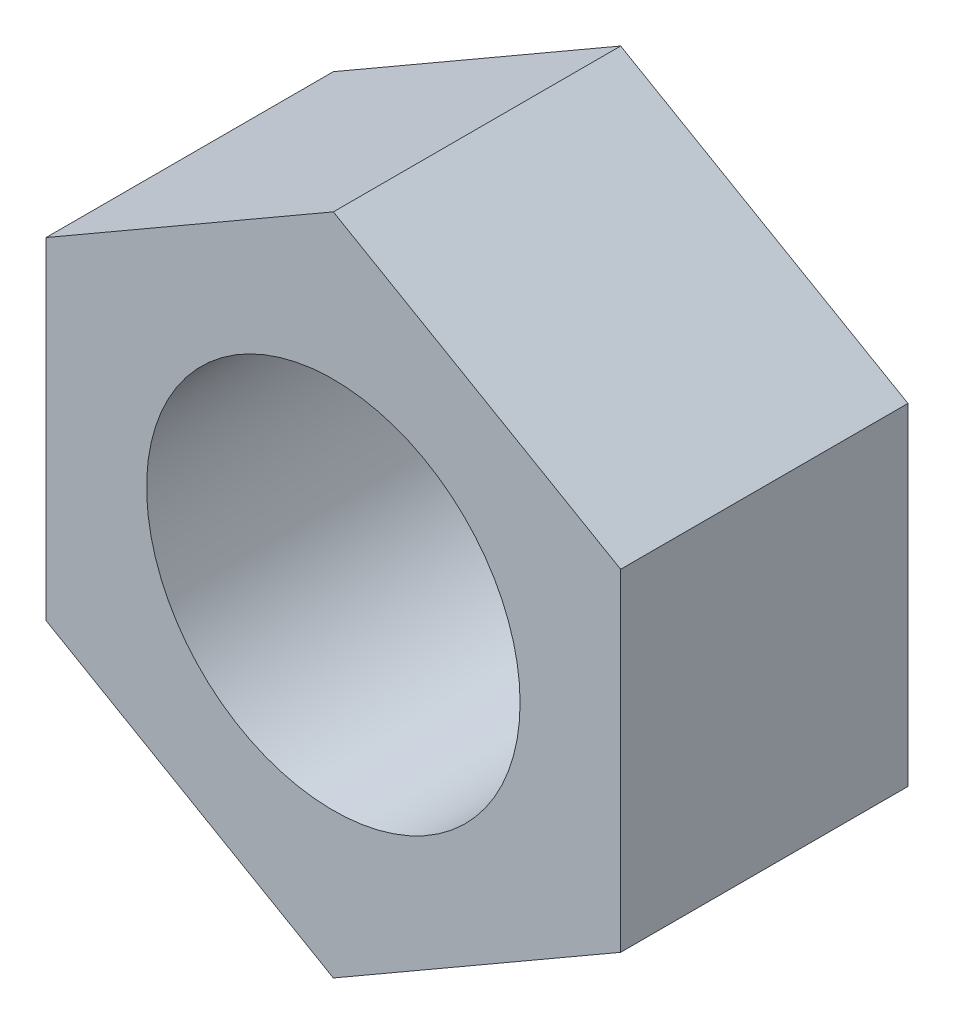
SolidWorks part; units mm, degrees
ref_plane "Front Plane" through (0, 0, 0) normal (0, 0, 1) x (1, 0, 0)
ref_plane "Top Plane" through (0, 0, 0) normal (0, 1, 0) x (1, 0, 0)
ref_plane "Right Plane" through (0, 0, 0) normal (1, 0, 0) x (0, 0, -1)
sketch "Sketch1" plane through (0, 0, 0) normal (0, 0, 1) x (1, 0, 0)
  line L1 (0, 9.2376) -> (-8, 4.6188)
  line L2 (-8, 4.6188) -> (-8, -4.6188)
  line L3 (-8, -4.6188) -> (0, -9.2376)
  line L4 (0, -9.2376) -> (8, -4.6188)
  line L5 (8, -4.6188) -> (8, 4.6188)
  line L6 (8, 4.6188) -> (0, 9.2376)
  circle A0 centre (0, 0) radius 8 construction
  circle A1 centre (0, 0) radius 5.2
extrude "Boss-Extrude1" add sketch "Sketch1" along normal blind 8
